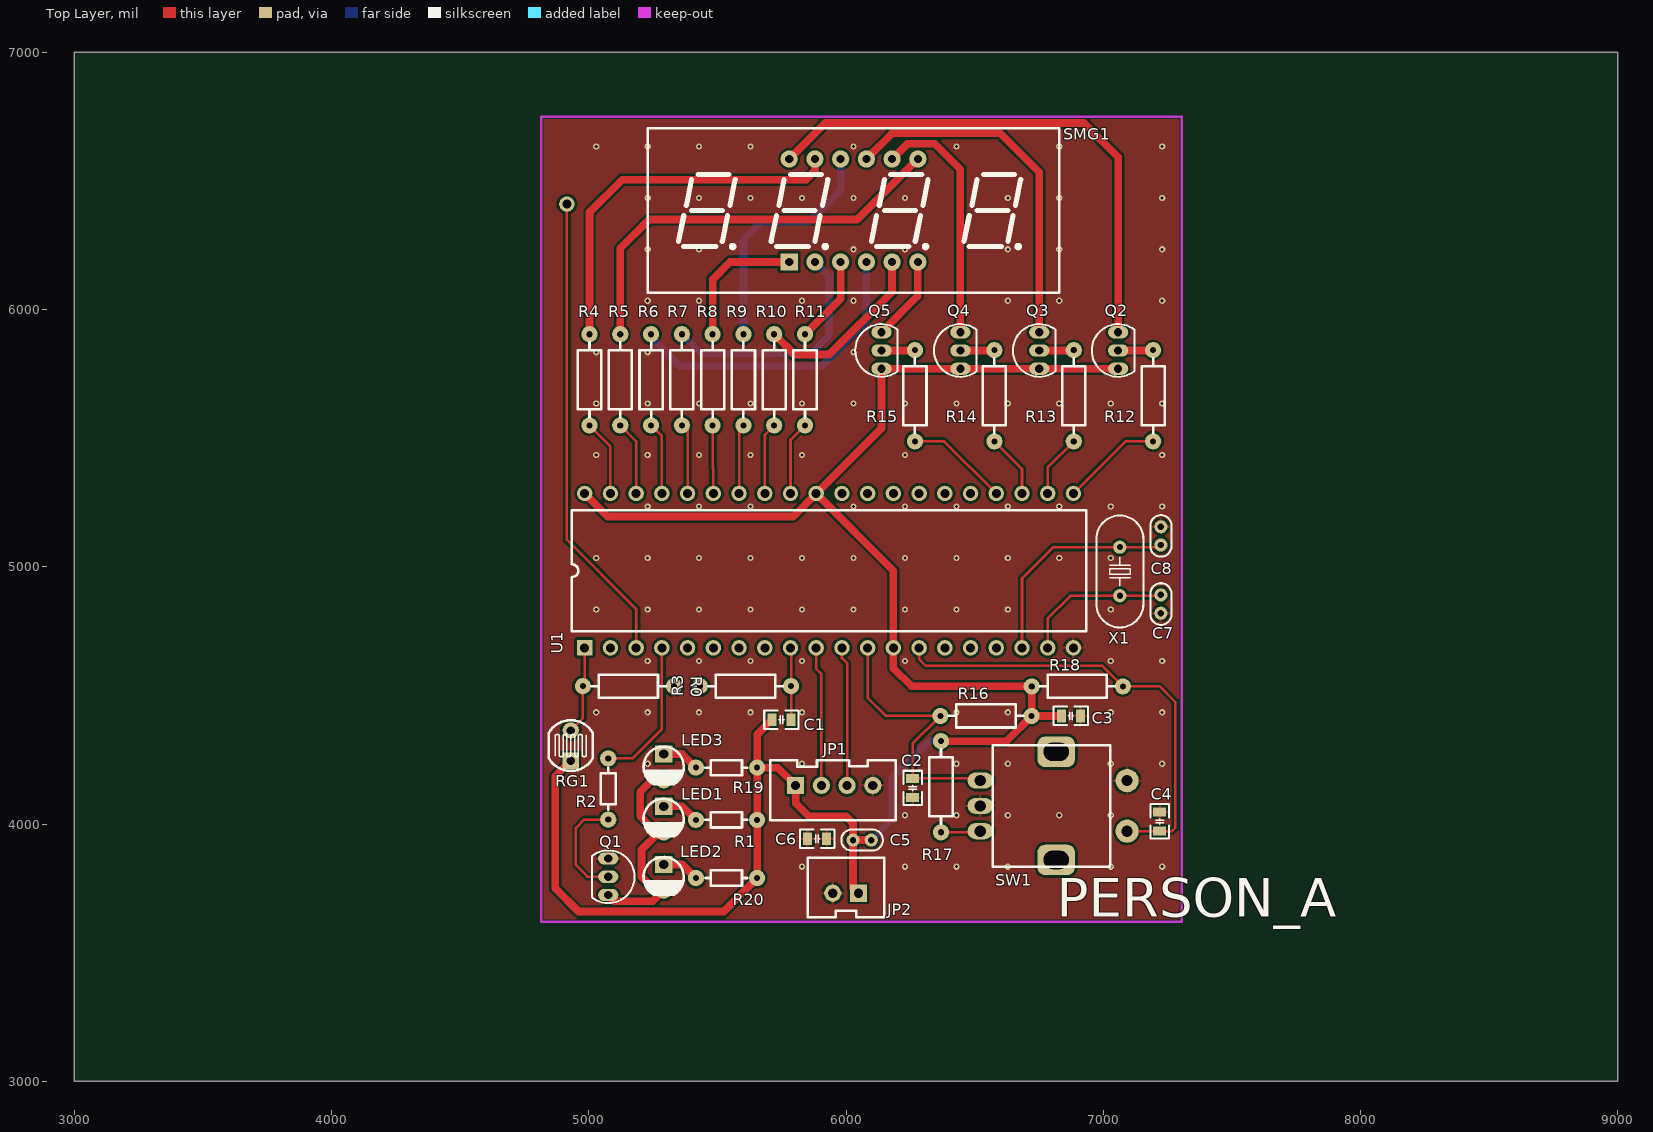
[diagram p0: Top Layer view]
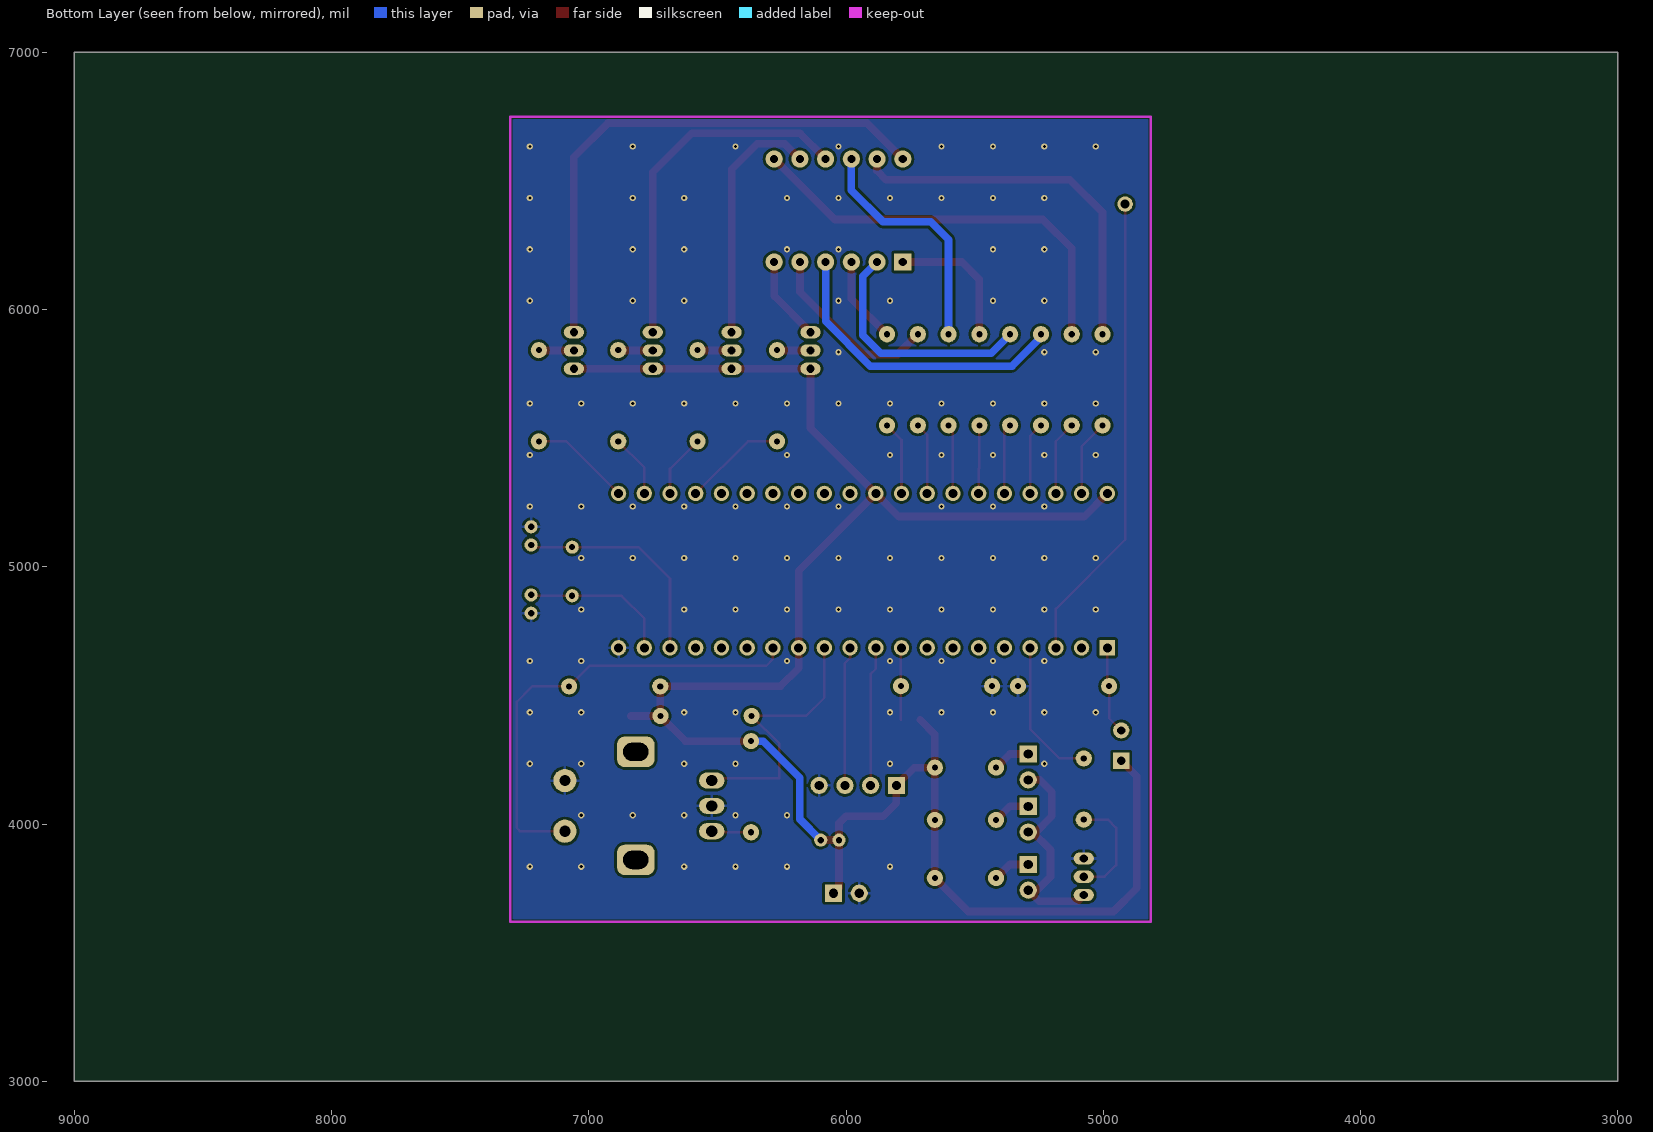
[diagram p1: Bottom Layer view, seen from below]
# Altium PCB MISC51984.pcbdoc
Units mil, origin at the board's own origin, x right, y up, seen from the top; angles counter-clockwise.
Board outline 6000 x 4000 mil, 2 copper layers (Top Layer, Bottom Layer); 44 components, 46 nets, 149 pads, 117 vias.

## Layer stack, top to bottom (the 12.6 mil dielectric is the usual default, probably not edited)
Top Solder Mask Layer: solder mask 0.4, Solder Resist, Dk 3.5
Top Layer: signal copper 1.4
Dielectric 1: surface 12.6, FR-4, Dk 4.8
Bottom Layer: signal copper 1.4
Bottom Solder Mask Layer: solder mask 0.4, Solder Resist, Dk 3.5

## Board outline
3000,7000 3000,3000 9000,3000 9000,7000

## Design rules (kind name [scope] priority, off if disabled: settings)
BoardOutlineClearance Clearance_1 [All] p2: genericclearance=10 ignorepadtopadclearanceinfootprint=FALSE except(0: Arc-SplitContinuation Track-SplitContinuation SMDPad-SplitContinuation THPad-SplitContinuation Via-SplitContinuation Fill-SplitContinuation Region-SplitContinuation Poly-SplitContinuation Text-SplitContinuation Hole-SplitContinuation; 6: SMDPad-CutoutEdge THPad-CutoutEdge Via-CutoutEdge Fill-CutoutEdge Region-CutoutEdge Text-CutoutEdge; 6.9: Hole-CutoutEdge; 10: Arc-OutlineEdge Track-OutlineEdge SMDPad-OutlineEdge THPad-OutlineEdge Via-OutlineEdge Fill-OutlineEdge Region-OutlineEdge Poly-OutlineEdge Text-OutlineEdge Hole-OutlineEdge Poly-CutoutEdge; 11.8: Arc-CutoutEdge Track-CutoutEdge)
Clearance [All] p1: gap=10 ignorepadtopadclearanceinfootprint=FALSE
DiffPairsRouting [All] p1: maxlimit=10 minlimit=6 mostfreqgap=6 toplayer_minwidth=15 toplayer_prefwidth=15 toplayer_maxwidth=15 toplayer_mingap=10 toplayer_prefgap=10 toplayer_maxgap=10 bottomlayer_minwidth=15 bottomlayer_prefwidth=15 bottomlayer_maxwidth=15 bottomlayer_mingap=10 bottomlayer_prefgap=10 bottomlayer_maxgap=10 maxuncoupledlength=10
HoleToHoleClearance ComponentClearance [All] p1: gap=10 allowstackedmicrovias=TRUE
Length netLength [All] p1: minlimit=0 maxlimit=0
MatchedLengths netLengthTolerance [All] p1: tolerance=1000
PolygonConnect [(InNet('GND'))] p1: connectstyle=Relief reliefconductorwidth=10 reliefentries=4 polygonreliefangle="90 Angle" airgapwidth=10 via.connectstyle=Relief via.reliefconductorwidth=10 via.reliefentries=4 via.polygonreliefangle="90 Angle" via.airgapwidth=10
RoutingVias [All] p1: holewidth=28 width=50 viastyle="Through Hole" minholewidth=1 minwidth=1 maxholewidth=28 maxwidth=50
SolderMaskExpansion [All] p1: expansion=4 istentingtop=FALSE
Width [All] p1: maxlimit=10 minlimit=10 preferedwidth=10 toplayer_minwidth=10 toplayer_maxwidth=17952.8 toplayer_prefwidth=10 bottomlayer_minwidth=10 bottomlayer_maxwidth=17952.8 bottomlayer_prefwidth=10
2 further rules are at their usual default settings.

## Components (designator, comment, footprint, x,y, rotation, side; value= is the part's Value field where it differs from the comment)
C1 "10uF" C0805_L 5749.2,4405.01 r180 top
C2 "0.1uF" C0805_L 6259.2,4140.01 r90 top
C3 "0.1uF" C0805_L 6874.2,4420.01 r0 top
C4 "0.1uF" C0805_L 7219.2,4010.01 r270 top
C5 "104" "CC 1.8*3.6" 6062.64,3937.58 r0 top
C6 "220uF" C0805_L 5887.64,3942.58 r180 top
C7 "22pF" "CC 1.8*3.6" 7224.2,4855.01 r90 top
C8 "22pF" "CC 1.8*3.6" 7224.2,5120.01 r270 top
JP1 "HDR-1X4" XH2.54-LI-4P 5954.2,4150.01 r0 top
JP2 "HDR-1X2" XH2.54-LI-2P 5998.45,3730.93 r180 top
LED1 "Red" "LED 3MM-B" 5291.55,4018.6 r270 top
LED2 "Red" "LED 3MM-B" 5291.55,3792.67 r270 top
LED3 "Red" "LED 3MM-B" 5291.55,4221.79 r270 top
Q1 "S9013" TO92A 5075.67,3795.01 r270 top
Q2 "S9012" TO92A 7058.02,5840.84 r90 top
Q3 "S9012" TO92A 6751.35,5840.84 r90 top
Q4 "S9012" TO92A 6444.69,5840.84 r90 top
Q5 "S9012" TO92A 6138.02,5840.84 r90 top
R0 "10K" AXIAL0.4-1/4W 5154.2,4535.79 r0 top
R1 "100" AXIAL0.3-1/8W 5536.55,4015.92 r0 top
R2 "1K" AXIAL0.3-1/8W 5075.67,4135.01 r270 top
R3 "10K" AXIAL0.4-1/4W 5609.2,4535.79 r180 top
R4 "220" AXIAL0.4-1/4W 5002.8,5726.85 r270 top
R5 "220" AXIAL0.4-1/4W 5122.49,5726.85 r90 top
R6 "220" AXIAL0.4-1/4W 5242.17,5726.85 r90 top
R7 "220" AXIAL0.4-1/4W 5361.86,5726.85 r90 top
R8 "220" AXIAL0.4-1/4W 5481.54,5726.85 r90 top
R9 "220" AXIAL0.4-1/4W 5601.23,5726.85 r90 top
R10 "220" AXIAL0.4-1/4W 5720.91,5726.85 r270 top
R11 "220" AXIAL0.4-1/4W 5840.6,5726.85 r90 top
R12 "1K" AXIAL0.4-1/4W 7194.2,5664.86 r90 top
R13 "1K" AXIAL0.4-1/4W 6885.47,5664.86 r90 top
R14 "1K" AXIAL0.4-1/4W 6576.75,5664.86 r90 top
R15 "1K" AXIAL0.4-1/4W 6268.02,5664.86 r90 top
R16 "10K" AXIAL0.4-1/4W 6544.2,4420.01 r0 top
R17 "10K" AXIAL0.4-1/4W 6369.2,4145.01 r270 top
R18 "10K" AXIAL0.4-1/4W 6899.2,4535.01 r180 top
R19 "100" AXIAL0.3-1/8W 5536.55,4219.11 r0 top
R20 "100" AXIAL0.3-1/8W 5536.55,3789.99 r0 top
RG1 "10K" RG5528 4930,4305 r90 top
SMG1 "4041B" "SMG 0.4-4P" 6029.2,6385.01 r0 top
SW1 "EC11" EC11-B 6807.19,4070.49 r180 top
U1 "STC12C5A60S2" DIP-40 4984.2,4685.01 r90 top
X1 "11.0592MHz" HC-49S 7064.5,4981.72 r270 top

## Footprints (in the part's own frame and the unit in brackets; to place one, negate y for a bottom-side part, rotate by r counter-clockwise, add the part's x,y. Pads: shape width x height; smd on the part's side, far side on the other; paste and mask are expansions set on the pad)
AXIAL0.3-1/8W [mm]
  round 1.6 hole 0.6: 1(-3.048,0) 2(3,0)
  silkscreen extent -2.1,-0.75 2,0.75
AXIAL0.4-1/4W [mm]
  round 1.6 hole 0.6: 1(-4.5,0) 2(4.5,0)
  silkscreen extent -3.68,-1.14 3.68,1.14
C0805_L [mil]
  rect 35x50 smd: 1(-37.4,0) 2(37.4,0)
  silkscreen extent -67,-36 67,36
"CC 1.8*3.6" [mm]
  round 1.3 hole 0.635: 1(-0.9,0) 2(0.9,0)
  silkscreen extent -2.05,-1.04 2.05,1.04
DIP-40 [mil]
  rect 60x60 hole 35: 1(0,0)
  round 60 hole 35: 2(0,-100) 3(0,-200) 4(0,-300) 5(0,-400) 6(0,-500) 7(0,-600) 8(0,-700) 9(0,-800) 10(0,-900) 11(0,-1000) 12(0,-1100) 13(0,-1200) 14(0,-1300) 15(0,-1400) 16(0,-1500) 17(0,-1600) 18(0,-1700) 19(0,-1800) 20(0,-1900) 21(600,-1900) 22(600,-1800) 23(600,-1700) 24(600,-1600) 25(600,-1500) 26(600,-1400) 27(600,-1300) 28(600,-1200) 29(600,-1100) 30(600,-1000) 31(600,-900) 32(600,-800) 33(600,-700) 34(600,-600) 35(600,-500) 36(600,-400) 37(600,-300) 38(600,-200) 39(600,-100) 40(600,0)
  silkscreen extent 65,-1950 535,50
EC11-B [mm]
  rrect50% 3.7x3 hole 1.8 slot 2.5 at 0 deg: 0(-0.254,5.334) 0(-0.254,-5.334)
  round 2.3 hole 1.1: 1(-7.25,2.5) 2(-7.25,-2.5)
  oval 2.5x1.6 hole 1.1: A(7.25,-2.5) B(7.25,2.5) C(7.25,0)
  silkscreen extent -5.59,-6 6,6
HC-49S [mm]
  round 1.3 hole 0.6: 1(-2.4,0) 2(2.4,0)
  silkscreen extent -5.52,-2.32 5.52,2.33
"LED 3MM-B" [mm]
  rect 1.7x1.7 hole 0.9: 1(-1.27,0)
  round 1.7 hole 0.9: 2(1.27,0)
  silkscreen extent -2.01,-2 1.72,1.98
RG5528 [mm]
  rect 1.6x1.6 hole 0.8: 1(-1.5,0)
  round 1.6 hole 0.8: 2(1.5,0)
  silkscreen extent -2.5,-2.16 2.5,2.16
"SMG 0.4-4P" [mm]
  rect 1.7x1.7 hole 0.8: 1(-6.35,-5.08)
  round 1.7 hole 0.8: 2(-3.81,-5.08) 3(-1.27,-5.08) 4(1.27,-5.08) 5(3.81,-5.08) 6(6.35,-5.08) 7(6.35,5.08) 8(3.81,5.08) 9(1.27,5.08) 10(-1.27,5.08) 11(-3.81,5.08) 12(-6.35,5.08)
  silkscreen extent -20.32,-8.13 20.32,8.13
TO92A [mm]
  oval 1.2x2 hole 0.8: 1(-1.8,0) 2(0,0) 3(1.8,0)
  silkscreen extent -2.6,-1.6 2.6,2.6
XH2.54-LI-2P [mm]
  rect 1.7x1.7 hole 0.9: 1(-1.27,0)
  round 1.7 hole 0.9: 2(1.27,0)
  silkscreen extent -3.81,-3.51 3.74,2.37
XH2.54-LI-4P [mm]
  rect 1.7x1.7 hole 0.9: 1(-3.81,0)
  round 1.7 hole 0.9: 2(-1.27,0) 3(1.27,0) 4(3.81,0)
  silkscreen extent -6.3,-3.45 6.07,2.49

## Free pads (board coordinates)
  round 60 hole 36: 1(4915,6410)

## Via types
v1: diameter 24, hole 12, Top Layer to Bottom Layer, 117 vias

## Nets (pads, with @x,y where several pads share a name; then routed paths per layer and width w, separated by ;. In a path a pad name is that pad's centre, name@x,y a point inside that pad or via, vN(x,y) a via of type N, cw(c..) or ccw(c..) an arc to the next point about the centre after c; other vN are vias at no path point)
$2N74: Q1.2 R2.2 | length 428.2
  Top Layer w10: Q1.2 4994.99,3795.01 4950,3840 4950,3985 4981.9,4016.9 R2.2
$2N75: LED1.2 LED2.2 LED3.2 Q1.3 | length 876.7
  Top Layer w30: Q1.3 5099.82,3700 5248.89,3700 LED2.2 5257.33,3742.67 5205,3795 5205,3900 LED1.2@5273.6,3968.6 ; LED1.2 LED1.2@5273.6,3968.6 ; LED3.2 5246.79,4171.79 5200,4125 5200,4030 5261.4,3968.6 LED1.2@5273.6,3968.6
$2N76: R4.1 SMG1.11 | length 1462.9
  Top Layer w30: R4.1 5002.8,6377.8 5130,6505 5845,6505 5879.2,6539.2 SMG1.11
$2N77: R6.2 SMG1.4 | length 1197.9
  Bottom Layer w30: R6.2 5242.17,5892.83 5355,5780 5905,5780 6079.2,5954.2 SMG1.4
$2N78: R7.2 SMG1.2 | length 940.9
  Bottom Layer w30: R7.2 5435.87,5830 5865,5830 5935,5900 5935,6129.21 SMG1.2
$2N79: R5.2 SMG1.7 | length 1634.1
  Top Layer w30: R5.2 5122.49,6237.49 5235,6350 6044.18,6350 SMG1.7
$2N80: R8.2 SMG1.1 | length 538.5
  Top Layer w30: R8.2 5481.54,6116.54 5550.01,6185.01 SMG1.1
$2N81: R9.2 SMG1.10 | length 945.9
  Bottom Layer w30: R9.2 5601.23,6271.23 5670.98,6340.98 5855.98,6340.98 5979.2,6464.2 SMG1.10
$2N82: R11.2 SMG1.3 | length 338.4
  Top Layer w30: R11.2 5979.2,6042.61 SMG1.3
$2N83: R10.1 SMG1.5 | length 708
  Top Layer w30: R10.1 5799.92,5825 5935,5825 6179.2,6069.2 SMG1.5
$2N84: Q2.2 R12.2 | length 136.7
  Top Layer w30: Q2.2 7193.02,5840.84 R12.2
$2N85: Q4.2 R14.2 | length 132.5
  Top Layer w30: Q4.2 6575.57,5840.84 R14.2
$2N86: Q5.2 R15.2 | length 130.5
  Top Layer w30: Q5.2 6266.84,5840.84 R15.2
$2N87: Q3.2 R13.2 | length 134.6
  Top Layer w30: Q3.2 6884.29,5840.84 R13.2
$2N88: R17.2 SW1.B | length 154.3
  Top Layer w10: R17.2 6517.54,3967.85 SW1.B
$2N89: LED1.1 R1.1 | length 146.8
  Top Layer w30: LED1.1 5363.88,4068.6 R1.1
$2N90: LED2.1 R20.1 | length 146.8
  Top Layer w30: LED2.1 5363.88,3842.67 R20.1
$2N91: LED3.1 R19.1 | length 146.8
  Top Layer w30: LED3.1 5363.88,4271.79 R19.1
A1: Q2.3 SMG1.12 | length 2072.2
  Top Layer w30: SMG1.12 5919.18,6725 6925,6725 7058.02,6591.98 Q2.3
A2: Q3.3 SMG1.9 | length 1398.2
  Top Layer w30: SMG1.9 6179.18,6685 6600,6685 6751.35,6533.65 Q3.3
A3: Q4.3 SMG1.8 | length 965.2
  Top Layer w30: SMG1.8 6239.18,6645 6345,6645 6444.69,6545.31 Q4.3
A4: Q5.3 SMG1.6 | length 331.8
  Top Layer w30: Q5.3 6279.2,6052.88 SMG1.6
DIG1: R12.1 U1.21 | length 394
  Top Layer w10: U1.21 7086.88,5487.69 R12.1
DIG2: R13.1 U1.22 | length 244.6
  Top Layer w10: U1.22 6784.2,5386.42 R13.1
DIG3: R14.1 U1.23 | length 247.2
  Top Layer w10: R14.1 6684.2,5380.24 U1.23
DIG4: R15.1 U1.24 | length 400.1
  Top Layer w10: R15.1 6381.52,5487.69 U1.24
EC11_A: C2.2 R16.1 SW1.A U1.12 | length 1059.7
  Top Layer w10: U1.12 6084.2,4490.8 6154.99,4420.01 R16.1 6259.2,4312.18 C2.2 6513.27,4177.41 SW1.A
EC11_KEY: C4.2 R18.1 SW1.1 U1.14 | length 1791.4
  Top Layer w10: U1.14 6284.2,4640.8 6310,4615 6996.38,4615 R18.1 7219.99,4535.01 7280,4475 7280,3985 7267.62,3972.62 C4.2 7218.65,3972.07 SW1.1
GND: C2.1 C3.2 C4.1 C6.1 C6.2 C7.1 C8.1 JP1.4 JP2.2 Q1.1 R0.2 R3.2 SW1.2 SW1.C U1.20
  other v1: 5829.1,3834.1 6229.1,3834.1 6429.1,3834.1 6629.1,3834.1 7029.1,3834.1 7229.1,3834.1 6229.1,4034.1 6429.1,4034.1 6629.1,4034.1 6829.1,4034.1 7029.1,4034.1 5229.1,4234.1 5829.1,4234.1 6429.1,4234.1 6629.1,4234.1 7029.1,4234.1 7229.1,4234.1 5029.1,4434.1 5229.1,4434.1 5429.1,4434.1 5629.1,4434.1 5829.1,4434.1 6429.1,4434.1 6629.1,4434.1 7029.1,4434.1 7229.1,4434.1 5229.1,4634.1 5429.1,4634.1 5629.1,4634.1 5829.1,4634.1 6229.1,4634.1 7029.1,4634.1 7229.1,4634.1 5029.1,4834.1 5229.1,4834.1 5429.1,4834.1 5629.1,4834.1 5829.1,4834.1 6029.1,4834.1 6229.1,4834.1 6429.1,4834.1 6629.1,4834.1 7029.1,4834.1 5029.1,5034.1 5229.1,5034.1 5429.1,5034.1 5629.1,5034.1 5829.1,5034.1 6029.1,5034.1 6229.1,5034.1 6429.1,5034.1 6629.1,5034.1 6829.1,5034.1 7029.1,5034.1 5229.1,5234.1 5429.1,5234.1 5629.1,5234.1 6029.1,5234.1 6229.1,5234.1 6429.1,5234.1 6629.1,5234.1 6829.1,5234.1 7029.1,5234.1 7229.1,5234.1 5029.1,5434.1 5229.1,5434.1 5429.1,5434.1 5629.1,5434.1 5829.1,5434.1 6229.1,5434.1 7229.1,5434.1 5029.1,5634.1 5229.1,5634.1 5429.1,5634.1 5629.1,5634.1 5829.1,5634.1 6029.1,5634.1 6229.1,5634.1 6429.1,5634.1 6629.1,5634.1 6829.1,5634.1 7029.1,5634.1 7229.1,5634.1 5029.1,5834.1 5229.1,5834.1 6029.1,5834.1 5229.1,6034.1 5429.1,6034.1 5829.1,6034.1 6029.1,6034.1 6629.1,6034.1 6829.1,6034.1 7229.1,6034.1 5229.1,6234.1 5429.1,6234.1 6029.1,6234.1 6229.1,6234.1 6629.1,6234.1 6829.1,6234.1 7229.1,6234.1 5229.1,6434.1 5429.1,6434.1 5629.1,6434.1 5829.1,6434.1 6029.1,6434.1 6229.1,6434.1 6629.1,6434.1 6829.1,6434.1 7229.1,6434.1 5029.1,6634.1 5229.1,6634.1 5429.1,6634.1 5629.1,6634.1 6029.1,6634.1 6429.1,6634.1 6829.1,6634.1 7229.1,6634.1
LDR_ADC: R0.1 RG1.2 U1.1 | length 343.4
  Top Layer w10: RG1.2 4977.04,4411.09 R0.1 4984.2,4542.95 U1.1
LED_PWM: R2.1 U1.4 | length 571.6
  Top Layer w10: R2.1 5170.01,4255.01 5284.2,4369.2 U1.4
MCU_RST: C1.1 R3.1 U1.9 | length 281
  Top Layer w10: U1.9 5786.37,4682.85 R3.1 5786.37,4405.26 C1.1
MCU_RXD: JP1.2 U1.10 | length 543.3
  Top Layer w10: U1.10 5884.2,4603.59 5904.2,4583.59 JP1.2
MCU_TXD: JP1.3 U1.11 | length 543.3
  Top Layer w10: U1.11 5984.2,4645.01 6004.2,4625.01 JP1.3
P12: pad.1 U1.3 | length 1836.5
  Top Layer w10: pad.1 4915,5105 5184.2,4835.8 U1.3
SEG_A: R4.2 U1.39 | length 298.4
  Top Layer w10: R4.2 5084.2,5468.28 U1.39
SEG_B: R5.1 U1.38 | length 290.2
  Top Layer w10: R5.1 5184.2,5487.97 U1.38
SEG_C: R6.1 U1.37 | length 282.1
  Top Layer w10: R6.1 5284.2,5507.65 U1.37
SEG_D: R7.1 U1.36 | length 273.9
  Top Layer w10: R7.1 5384.2,5527.34 U1.36
SEG_DP: R11.1 U1.32 | length 288
  Top Layer w10: U1.32 5784.2,5493.28 R11.1
SEG_E: R8.1 U1.35 | length 265.8
  Top Layer w10: R8.1 5481.54,5383.92 5484.2,5381.26 U1.35
SEG_F: R9.1 U1.34 | length 271.7
  Top Layer w10: U1.34 5584.2,5532.65 R9.1
SEG_G: R10.2 U1.33 | length 279.9
  Top Layer w10: U1.33 5684.2,5512.97 R10.2
VCC: C1.2 C3.1 C5.1 C5.2 JP1.1 JP2.1 Q2.1 Q3.1 Q4.1 Q5.1 R1.2 R16.2 R17.1 R18.2 R19.2 R20.2 RG1.1 U1.13 U1.31 U1.40 | length 7892.6
  Top Layer w30: RG1.1 4870,4185.94 4870,3750 4960,3660 5524.67,3660 R20.2 R1.2 R19.2 ; U1.40 5074.21,5195 5794.19,5195 U1.31 ; C1.2 5654.66,4347.88 R19.2 ; JP2.1 6027.2,3752.18 C5.1 ; C5.2 C5.1 ; R17.1 6623.53,4322.18 R16.2 ; C3.1 R16.2 ; Q2.1 Q3.1 Q4.1 Q5.1 6138.02,5538.83 U1.31 ; R19.2 5735.11,4219.11 JP1.1 5804.2,4080.8 5855,4030 6000,4030 6027.2,4002.8 C5.1 ; U1.31 6184.2,4985.01 U1.13 6184.2,4605.8 6254.99,4535.01 R18.2 6722.04,4420.68 R16.2
  Bottom Layer w30: C5.2 6180,4019.51 6180,4180 6322.18,4322.18 R17.1
XTAL1: C7.2 U1.19 X1.2 | length 592
  Top Layer w10: U1.19 6784.2,4799.2 6872.24,4887.24 X1.2 7220.99,4887.24 C7.2
XTAL2: C8.2 U1.18 X1.1 | length 863.2
  Top Layer w10: U1.18 6684.2,4954.2 6806.21,5076.21 X1.1 7215.83,5076.21 C8.2
pads on no net: SW1.0 U1.2 U1.5 U1.6 U1.7 U1.8 U1.15 U1.16 U1.17 U1.25 U1.26 U1.27 U1.28 U1.29 U1.30

## Polygon pours and split planes (outlines as drawn)
GND on Top Layer (solid, remove dead copper, pour order 0): 4550,6955 4550,3500 7550,3500 7550,6955
GND on Bottom Layer (solid, remove dead copper, pour order 2): 4625,6830 4625,3460 7455,3460 7455,6830

## Keep-outs
Board Outline Layer:
  lines w10: 4815,3620 4815,6750 7305,6750 7305,3620 4815,3620

## Silkscreen, mask and mechanical layers (free items; w line width, h text height)
Top Silkscreen Layer:
  text "PERSON_A" at 6820,3640 h150